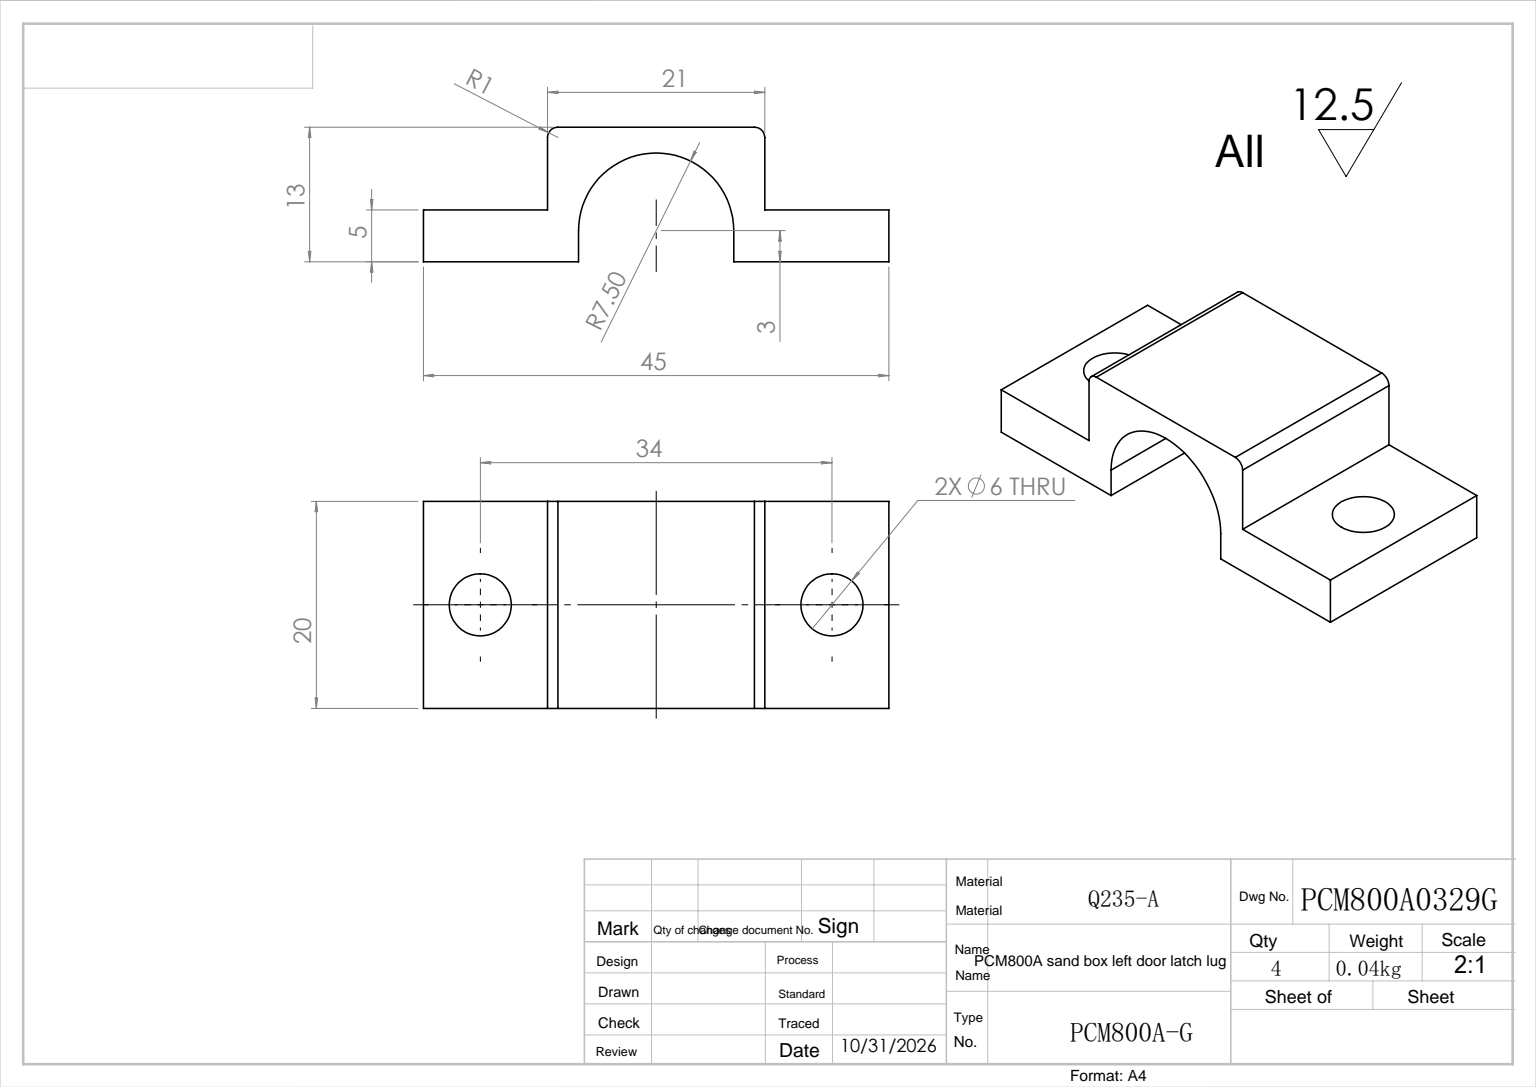
from build123d import *

# Parameters (mm, degrees)
EXTRUDE_1_DEPTH     = 20
FILLET_1_R          = 1
SKETCH_2_R          = 3
CUT_EXTRUDE_1_DEPTH = 50.889878733


with BuildPart() as part:
    # 草图1 → 凸台-拉伸1 (new body)
    with BuildSketch(Plane.XY):
        with BuildLine():
            Line((0, 0), (12, 0))
            Line((12, 0), (12, 8))
            Line((12, 8), (33, 8))
            Line((33, 8), (33, 0))
            Line((33, 0), (45, 0))
            Line((45, 0), (45, -5))
            Line((45, -5), (30, -5))
            Line((30, -5), (30, -2))
            ThreePointArc((30, -2), (22.5, 5.5), (15, -2))
            Line((15, -2), (15, -5))
            Line((15, -5), (0, -5))
            Line((0, -5), (0, 0))
        make_face()
    extrude(amount=EXTRUDE_1_DEPTH)

    # 圆角1
    fillet_1_edges = [part.edges().sort_by_distance(p)[0] for p in [
        (12, 8, 10),
        (33, 8, 10),
    ]]
    fillet(fillet_1_edges, radius=FILLET_1_R)

    # 草图2 → 切除-拉伸1 (cut, through all)
    with BuildSketch(Plane(origin=(0, 0, 0), x_dir=(1, 0, 0), z_dir=(0, 1, 0))):
        with Locations(Location((5.5, -10, 0), (0, 0, 270))):
            Circle(SKETCH_2_R)
        with Locations(Location((39.5, -10, 0), (0, 0, 270))):
            Circle(SKETCH_2_R)
    extrude(amount=-CUT_EXTRUDE_1_DEPTH, mode=Mode.SUBTRACT)


solid = part.part
